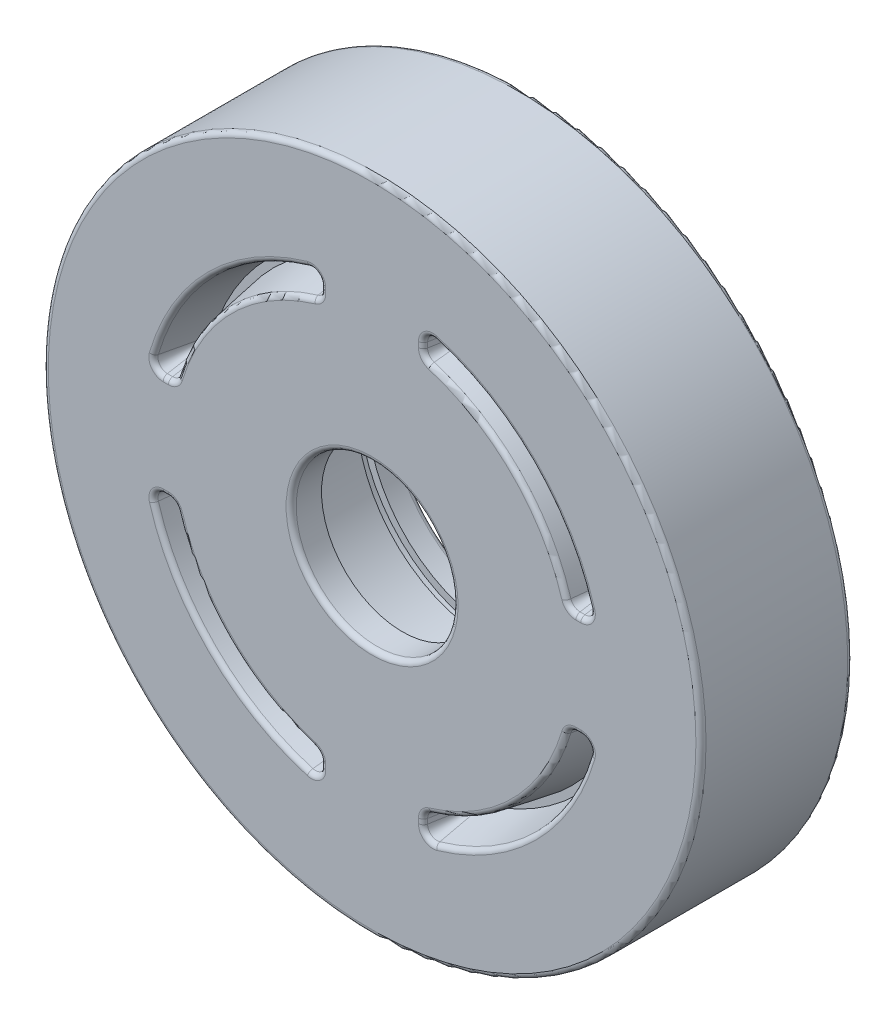
SolidWorks part; units mm, degrees
ref_plane "Front Plane" through (0, 0, 0) normal (0, 0, 1) x (1, 0, 0)
ref_plane "Top Plane" through (0, 0, 0) normal (0, 1, 0) x (1, 0, 0)
ref_plane "Right Plane" through (0, 0, 0) normal (1, 0, 0) x (0, 0, -1)
sketch "Sketch1" plane through (0, 0, 0) normal (0, 0, 1) x (1, 0, 0)
  circle A0 centre (0, 0) radius 65
  dimension "D1" = 130
extrude "Boss-Extrude1" add sketch "Sketch1" along normal mid plane 30
sketch "Sketch2" plane through (0, 0, 15) normal (0, 0, 1) x (1, 0, 0)
  circle A0 centre (0, 0) radius 16
  dimension "D1" = 32
extrude "Cut-Extrude1" cut sketch "Sketch2" against normal blind 6
sketch "Sketch3" plane through (0, 0, 9) normal (0, 0, 1) x (1, 0, 0)
  circle A0 centre (0, 0) radius 22.5
  dimension "D1" = 45
extrude "Cut-Extrude2" cut sketch "Sketch3" against normal blind 2
sketch "Sketch4" plane through (0, 0, 7) normal (0, 0, 1) x (1, 0, 0)
  circle A0 centre (0, 0) radius 26
  dimension "D1" = 52
extrude "Cut-Extrude3" cut sketch "Sketch4" against normal blind 15
sketch "Sketch5" plane through (0, 0, -8) normal (0, 0, 1) x (1, 0, 0)
  circle A0 centre (0, 0) radius 27.5
  dimension "D1" = 55
extrude "Cut-Extrude4" cut sketch "Sketch5" against normal blind 2
sketch "Sketch6" plane through (0, 0, -10) normal (0, 0, 1) x (1, 0, 0)
  circle A0 centre (0, 0) radius 26
  dimension "D1" = 52
extrude "Cut-Extrude5" cut sketch "Sketch6" against normal through all
fillet "Fillet1" radius 1 2 edges at (65, 0, -15) (65, 0, 15)
sketch "Sketch7" plane through (0, 0, -15) normal (0, 0, -1) x (-1, 0, 0)
  line L1 (-10, 40.2492) -> (-10, 41.2916)
  line L7 (-40.2749, 10) -> (-41.2458, 10)
  arc A0 (-11.4286, 38.3326) -> (-38.3256, 11.452) centre (0, 0) ccw
  arc A1 (-12.5581, 43.2122) -> (-43.1988, 12.6043) centre (0, 0) ccw
  arc A2 (-11.4286, 38.3326) -> (-10, 40.2492) centre (-12, 40.2492) ccw
  arc A3 (-10, 41.2916) -> (-12.5581, 43.2122) centre (-12, 41.2916) ccw
  arc A4 (-38.3256, 11.452) -> (-40.2749, 10) centre (-40.2749, 12.0344) cw
  arc A5 (-41.2458, 10) -> (-43.1988, 12.6043) centre (-41.2458, 12.0344) cw
  point P4 (0, 31.5736)
  point P5 (0, 50.591)
  point P9 (10, 31.5736)
  point P10 (10, 50.591)
  point P27 (0, 0)
  dimension "D1" = 80
  dimension "D2" = 90
  dimension "D3" = 2
  dimension "D4" = 2.0344
extrude "Cut-Extrude6" cut sketch "Sketch7" against normal blind 10 draft 10
pattern_circular "CirPattern1" count 4 over 360 about axis through (0, 0, 0) along (0, 0, 1) of "Cut-Extrude6"
mirror "Mirror1" about plane through (0, 0, 0) normal (0, 0, 1) of "CirPattern1", "Cut-Extrude6"
fillet "Fillet2" radius 1 66 edges at (-10.4029, 39.0596, 15) (-10, 40.7603, 15) (-10.8139, 42.8734, 15) (-31.8368, 31.8028, 15) (-42.8911, 10.7992, 15) (-40.7704, 10, 15) (-39.054, 10.3964, 15) (-28.2929, 28.2756, 15) (10.4029, -39.0596, 15) (10, -40.7603, 15) (10.8139, -42.8734, 15) (31.8368, -31.8028, 15) (42.8911, -10.7992, 15) (40.7704, -10, 15) (39.054, -10.3964, 15) (28.2929, -28.2756, 15) (16, 0, 15) (39.0596, 10.4029, 15) (40.7603, 10, 15) (42.8734, 10.8139, 15) (31.8028, 31.8368, 15) (10.7992, 42.8911, 15) (10, 40.7704, 15) (10.3964, 39.054, 15) (28.2756, 28.2929, 15) (-39.0596, -10.4029, 15) (-40.7603, -10, 15) (-42.8734, -10.8139, 15) (-31.8028, -31.8368, 15) (-10.7992, -42.8911, 15) (-10, -40.7704, 15) (-10.3964, -39.054, 15) (-28.2756, -28.2929, 15) (26, 0, -15) (10.7992, 42.8911, -15) (31.8028, 31.8368, -15) (42.8734, 10.8139, -15) (40.7603, 10, -15) (39.0596, 10.4029, -15) (28.2756, 28.2929, -15) (10.3964, 39.054, -15) (10, 40.7704, -15) (42.8911, -10.7992, -15) (31.8368, -31.8028, -15) (10.8139, -42.8734, -15) (10, -40.7603, -15) (10.4029, -39.0596, -15) (28.2929, -28.2756, -15) (39.054, -10.3964, -15) (40.7704, -10, -15) (-10.7992, -42.8911, -15) (-31.8028, -31.8368, -15) (-42.8734, -10.8139, -15) (-40.7603, -10, -15) (-39.0596, -10.4029, -15) (-28.2756, -28.2929, -15) (-10.3964, -39.054, -15) (-10, -40.7704, -15) (-42.8911, 10.7992, -15) (-31.8368, 31.8028, -15) (-10.8139, 42.8734, -15) (-10, 40.7603, -15) (-10.4029, 39.0596, -15) (-28.2929, 28.2756, -15) (-39.054, 10.3964, -15) (-40.7704, 10, -15)
sketch "Sketch8" plane through (0, 0, -15) normal (0, 0, -1) x (-1, 0, 0)
  circle A1 centre (0, 32.5) radius 1.5
  circle A2 centre (28.1458, -16.25) radius 1.5
  circle A3 centre (-28.1458, -16.25) radius 1.5
  point P11 (0, 0)
  dimension "D2" = 3
  dimension "D3" = 3
extrude "Cut-Extrude7" cut sketch "Sketch8" against normal blind 10
